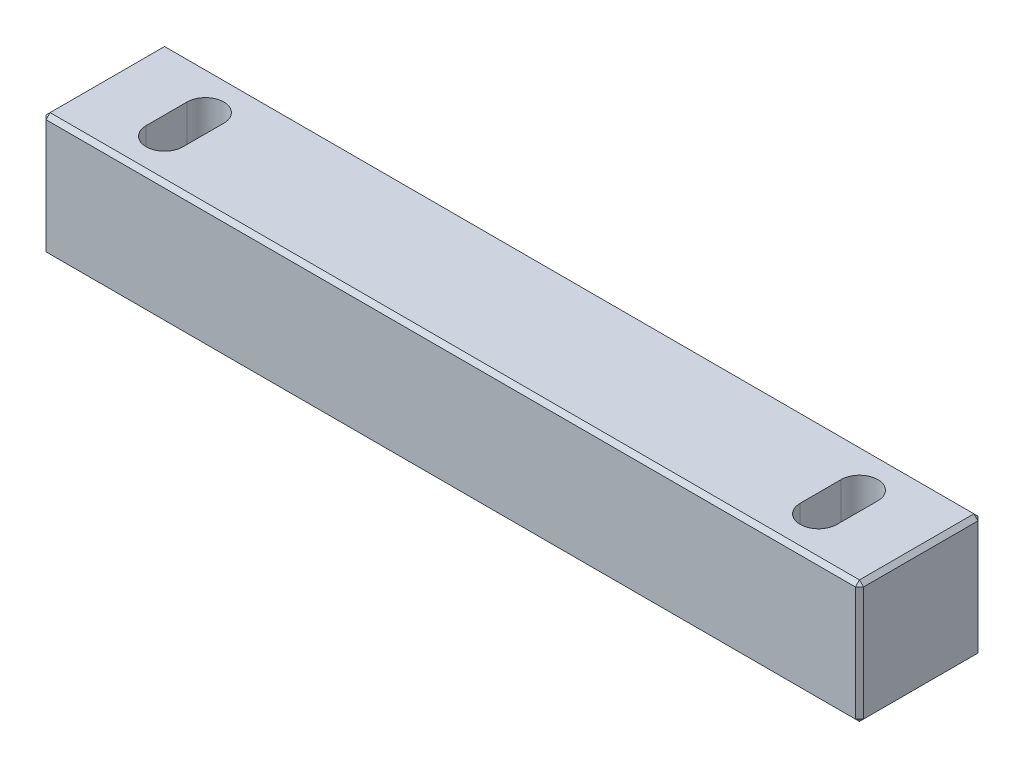
from build123d import *

# Parameters (mm, degrees)
SKETCH1_W          = 100
SKETCH1_H          = 15
EXTRUDE1_DEPTH     = 15
CUT_EXTRUDE1_DEPTH = 53.737557774
CHAMFER1_SIZE      = 0.5


with BuildPart() as part:
    # Sketch1 → Extrude1 (new body)
    with BuildSketch(Plane(origin=(0, 0, 0), x_dir=(1, 0, 0), z_dir=(0, 1, 0))):
        Rectangle(SKETCH1_W, SKETCH1_H)
    extrude(amount=EXTRUDE1_DEPTH)

    # Sketch4 → Cut-Extrude1 (cut, through all)
    with BuildSketch(Plane(origin=(0, 15, 0), x_dir=(1, 0, 0), z_dir=(0, 1, 0))):
        with BuildLine():
            Line((-42.25, 2.5), (-42.25, -2.5))
            ThreePointArc((-42.25, -2.5), (-40, -4.75), (-37.75, -2.5))
            Line((-37.75, -2.5), (-37.75, 2.5))
            ThreePointArc((-37.75, 2.5), (-40, 4.75), (-42.25, 2.5))
        make_face()
        with BuildLine():
            Line((37.75, 2.5), (37.75, -2.5))
            ThreePointArc((37.75, -2.5), (40, -4.75), (42.25, -2.5))
            Line((42.25, -2.5), (42.25, 2.5))
            ThreePointArc((42.25, 2.5), (40, 4.75), (37.75, 2.5))
        make_face()
    extrude(amount=-CUT_EXTRUDE1_DEPTH, mode=Mode.SUBTRACT)

    # Chamfer1
    chamfer1_edges = [part.edges().sort_by_distance(p)[0] for p in [
        (50, 15, 0),
        (0, 15, -7.5),
        (-50, 15, 0),
        (0, 0, -7.5),
        (50, 0, 0),
        (0, 0, 7.5),
        (-50, 0, 0),
        (0, 15, 7.5),
        (-50, 7.5, -7.5),
        (50, 7.5, -7.5),
        (50, 7.5, 7.5),
        (-50, 7.5, 7.5),
    ]]
    chamfer(chamfer1_edges, length=CHAMFER1_SIZE)


solid = part.part
